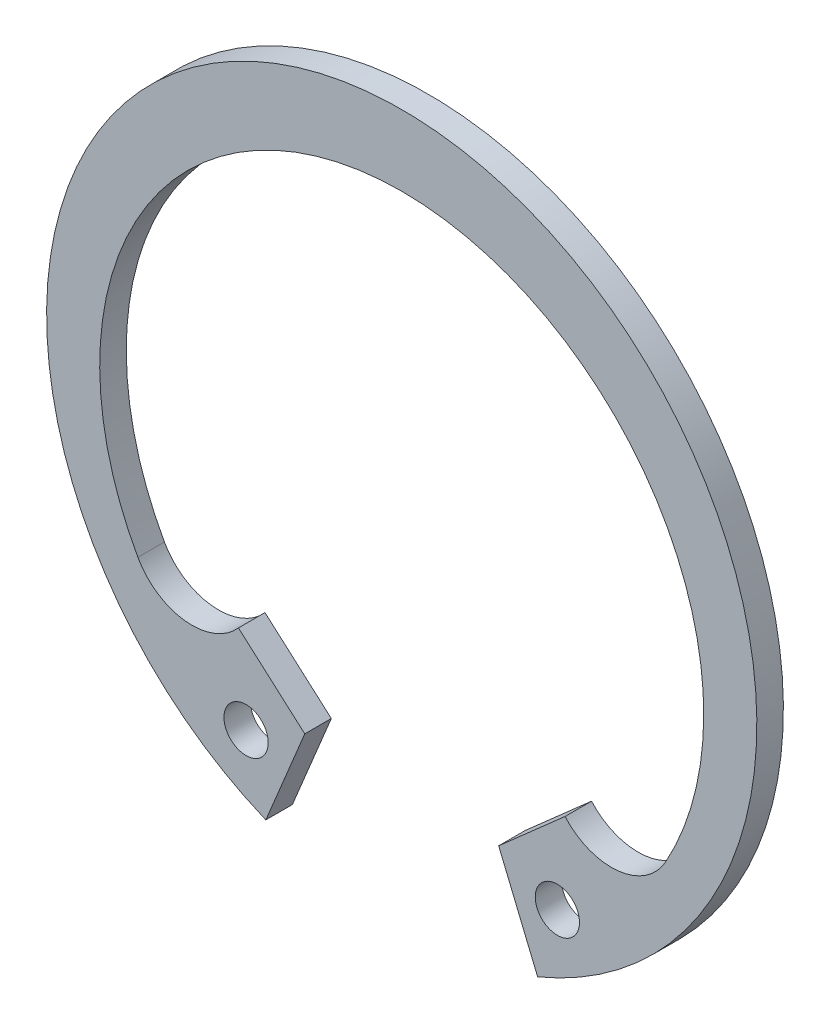
from build123d import *

# Parameters (mm, degrees)
SKETCH_1_R        = 1
EXTRUDE_952_DEPTH = 1.2


with BuildPart() as part:
    # 草图1 → Extrude 952 (new body)
    with BuildSketch(Plane.XY):
        with BuildLine():
            Line((-7.380473645, -7.931250769), (-4.381725301, -10.578420647))
            Line((-4.381725301, -10.578420647), (-6.142069089, -14.828266497))
            ThreePointArc((-6.142069089, -14.828266497), (0, 16.05), (6.142069089, -14.828266497))
            Line((6.142069089, -14.828266497), (4.381725301, -10.578420647))
            Line((4.381725301, -10.578420647), (7.380473645, -7.931250769))
            ThreePointArc((7.380473645, -7.931250769), (9.780239262, -8.8620448), (11.925945225, -7.440356203))
            ThreePointArc((11.925945225, -7.440356203), (0, 12.85), (-11.925945225, -7.440356203))
            ThreePointArc((-11.925945225, -7.440356203), (-9.780239262, -8.8620448), (-7.380473645, -7.931250769))
        make_face()
        with Locations((-7.034355028, -11.756183451)):
            Circle(SKETCH_1_R, mode=Mode.SUBTRACT)
        with Locations(Location((7.034355028, -11.756183451, 0), (0, 0, 180))):
            Circle(SKETCH_1_R, mode=Mode.SUBTRACT)
    extrude(amount=EXTRUDE_952_DEPTH)


solid = part.part
